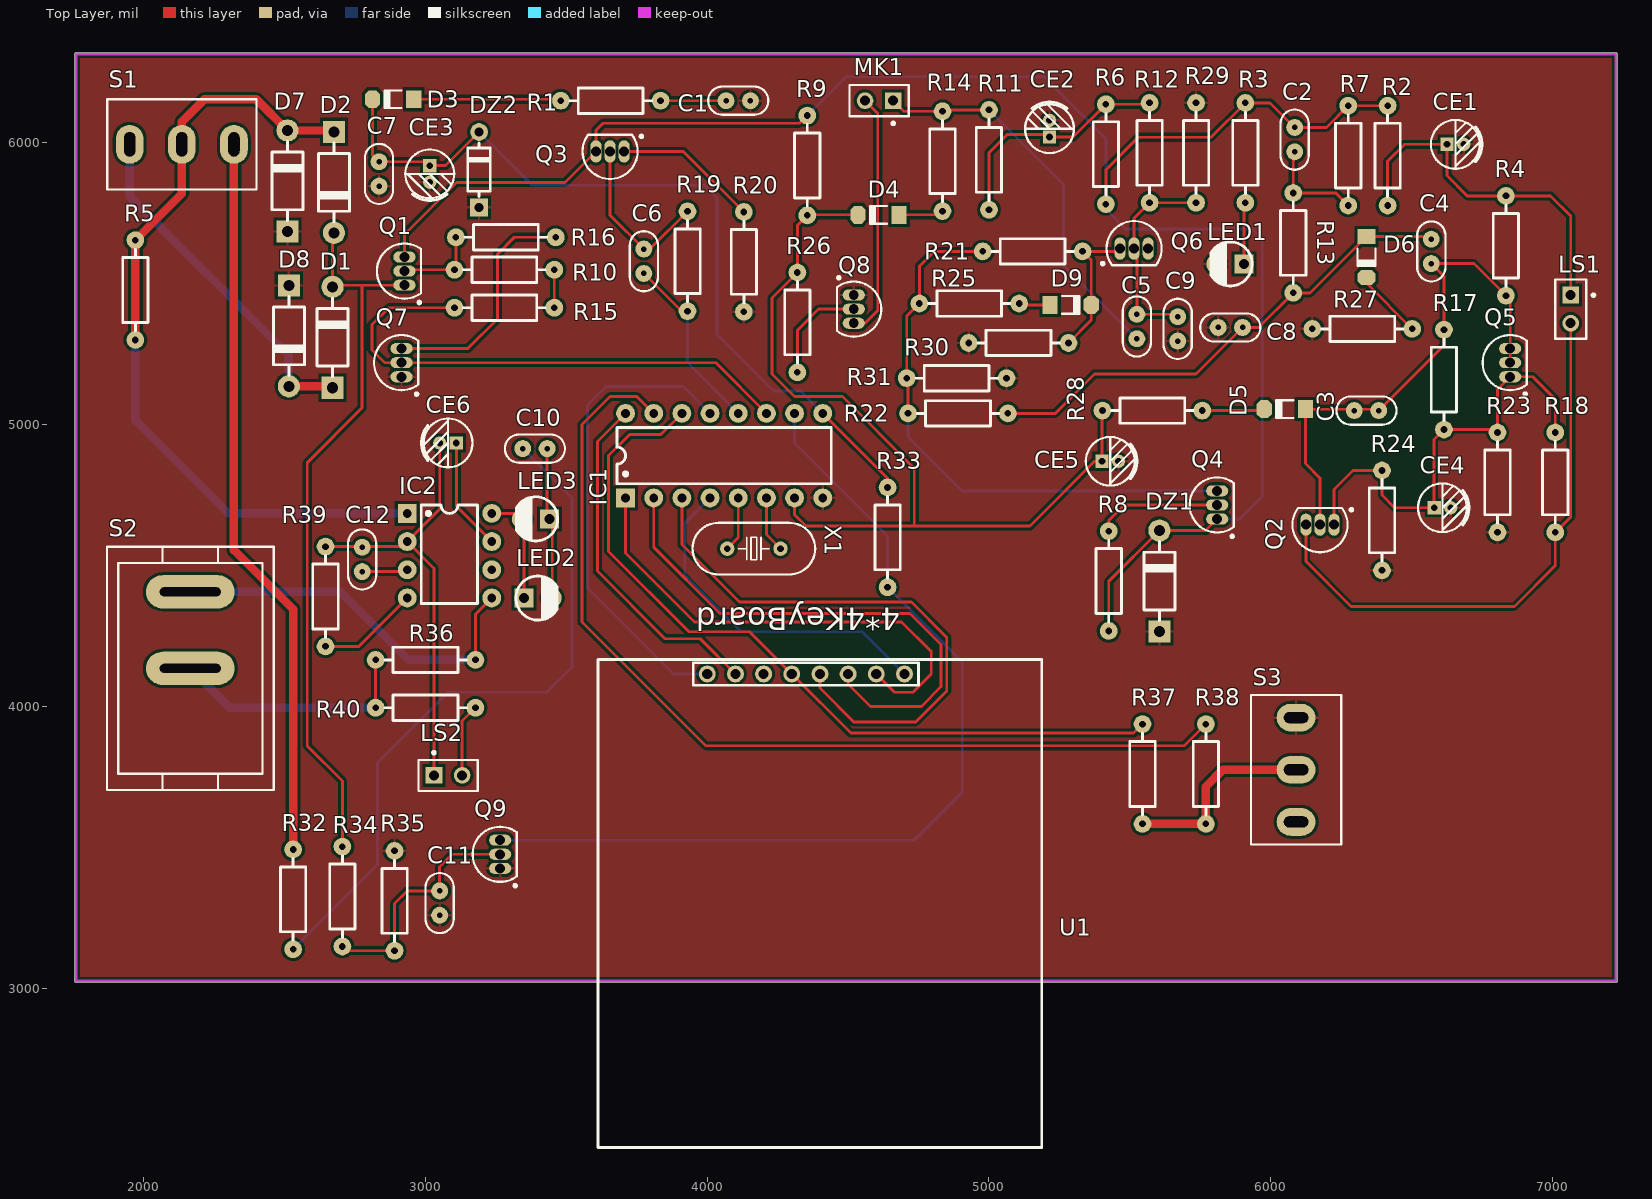
[diagram p0: Top Layer view]
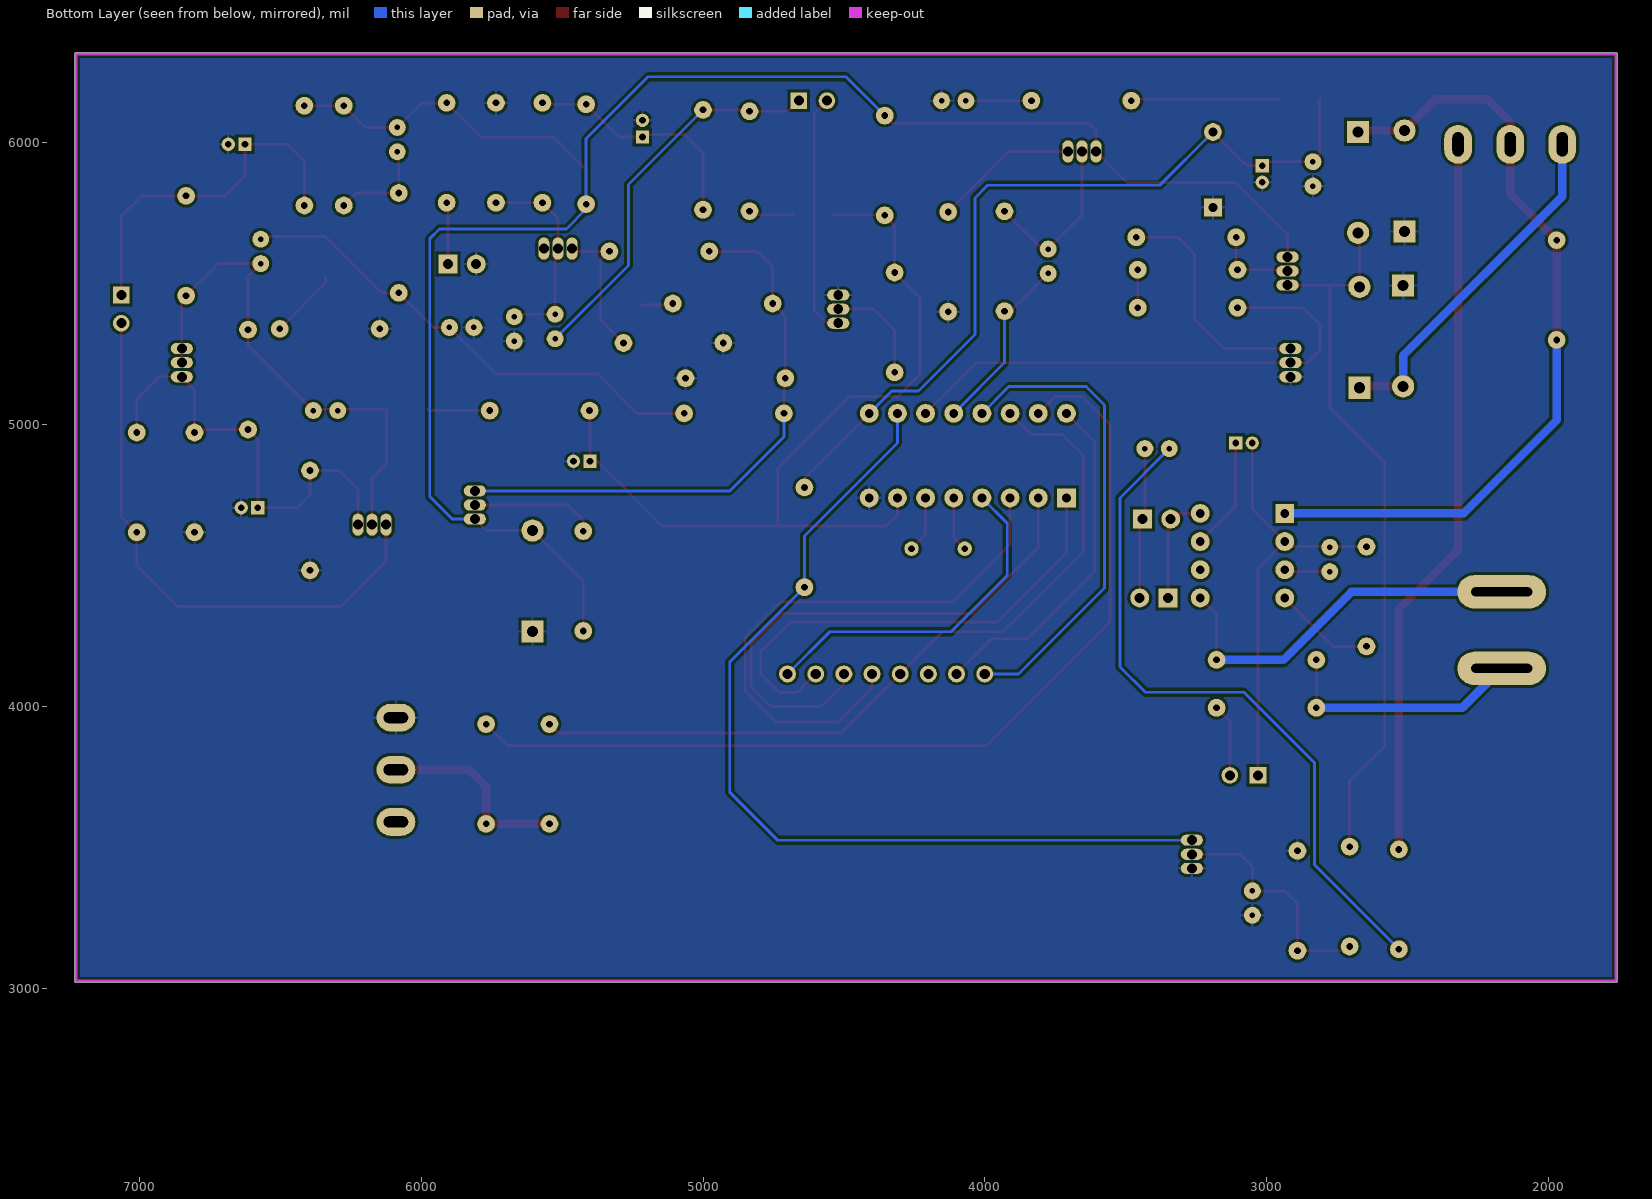
[diagram p1: Bottom Layer view, seen from below]
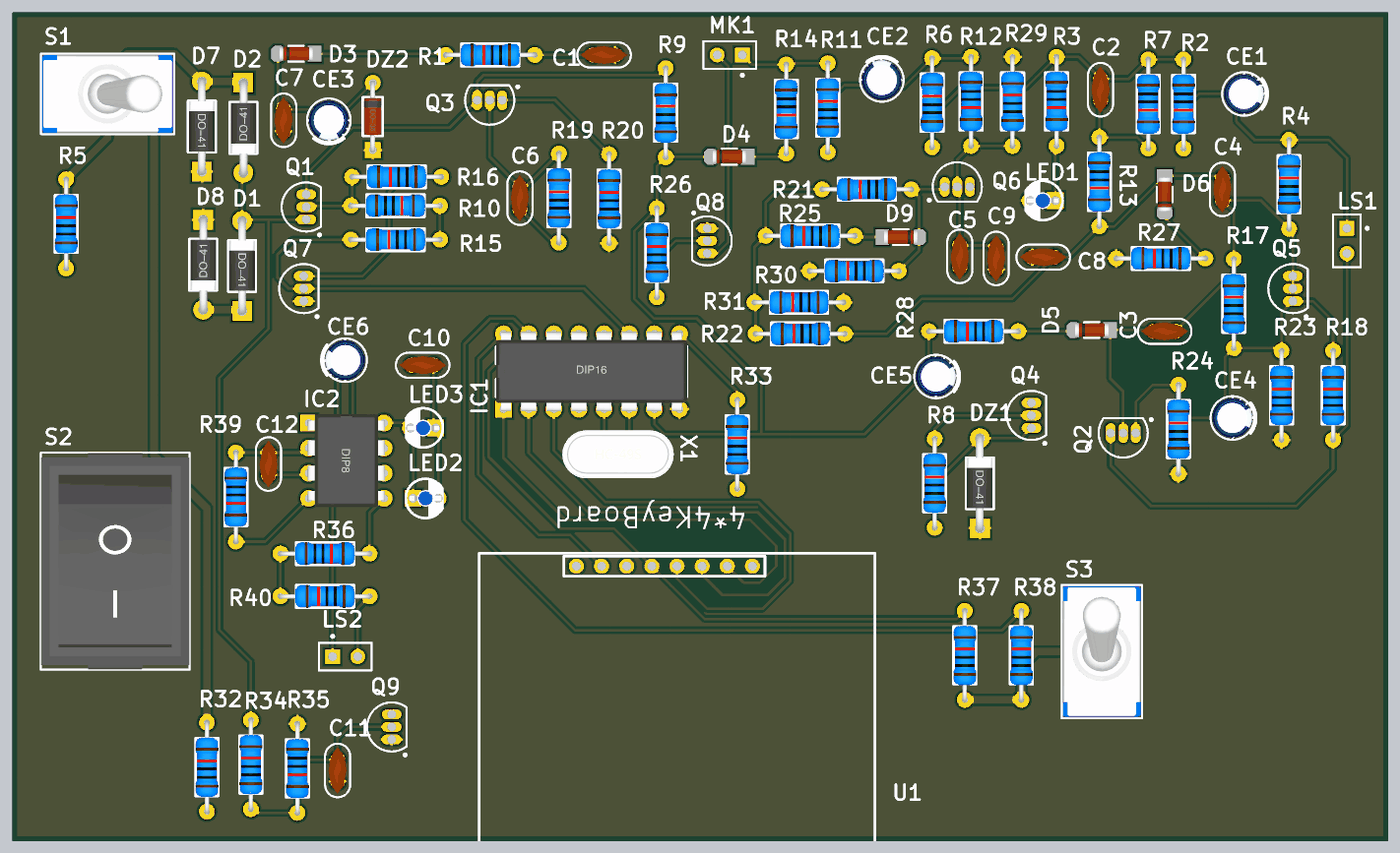
[diagram p2: 3D render of the assembled board from above, using the file's embedded part models]
# Altium PCB MISC82217.PcbDoc
Units mil, origin at the board's own origin, x right, y up, seen from the top; angles counter-clockwise.
Board outline 5475.03 x 3300.03 mil, 2 copper layers (Top Layer, Bottom Layer); 91 components, 60 nets, 219 pads, 0 vias.

## Layer stack, top to bottom (the 12.6 mil dielectric is the usual default, probably not edited)
Top Solder: solder mask 0.4, Solder Resist, Dk 3.5
Top Layer: signal copper 1.4
Dielectric 1: dielectric 12.6, FR-4, Dk 4.8
Bottom Layer: signal copper 1.4
Bottom Solder: solder mask 0.4, Solder Resist, Dk 3.5

## Board outline
1760,3019.99 cw(c1760,3025) 1754.98,3025 1754.98,6315 cw(c1760,6315) 1760,6320.02 7225,6320.02 cw(c7225,6315) 7230.02,6315 7230.02,3025 cw(c7225,3025) 7225,3019.99

## Design rules (kind name [scope] priority, off if disabled: settings)
Clearance [All] p1: gap=10
Height [All] p1: minheight=0 maxheight=99999 prefheight=500
HoleSize [All] p1: absolutevalues=TRUE maxlimit=1000 minlimit=1 maxpercent=80.000 minpercent=20.000
MinimumSolderMaskSliver [All] p1: minsoldermaskwidth=0
PolygonConnect [All] p1: connectstyle=Relief reliefconductorwidth=10 reliefentries=4 polygonreliefangle="90 Angle" airgapwidth=10
RoutingVias [All] p1: holewidth=28 width=50 viastyle="Through Hole" minholewidth=28 minwidth=50 maxholewidth=28 maxwidth=50
SilkToSilkClearance [All] p1: silktosilkclearance=0
SilkToSolderMaskClearance [IsPad] p1: minsilkscreentomaskgap=0 clearancetoexposedcopper=TRUE
SolderMaskExpansion [All] p1: expansion=4
Width [All] p1: maxlimit=30 minlimit=10 preferedwidth=10
25 further rules are at their usual default settings.

## Components (designator, comment, footprint, x,y, rotation, side; value= is the part's Value field where it differs from the comment)
C1 "22NF" "CC 2.2*5" 4110,6150 r180 top
C2 "10NF" "CC 2.2*5" 6085,6011.69 r90 top
C3 "100NF" "CC 2.2*5" 6340,5050 r180 top
C4 "100NF" "CC 2.2*5" 6570,5615 r90 top
C5 "10NF" "CC 2.2*5" 5525,5348.31 r270 top
C6 "22NF" "CC 2.2*5" 3775,5580 r90 top
C7 "100NF" "CC 2.2*5" 2835,5890 r90 top
C8 "22NF" "CC 2.2*5" 5856.69,5345 r0 top
C9 "33NF" "CC 2.2*5" 5670,5340 r90 top
C10 "1UF" "CC 2.2*5" 3388.31,4915 r0 top
C11 "100NF" "CC 2.2*5" 3050,3301.69 r90 top
C12 "100NF" "CC 2.2*5" 2775,4521.69 r270 top
CE1 "100UF" "CAP 1.5*4*8" 6655.47,5995 r0 top
CE2 "4.7UF" "CAP 1.5*4*8" 5215,6050.47 r90 top
CE3 "100UF" "CAP 1.5*4*8" 3015,5890 r270 top
CE4 "47UF" "CAP 1.5*4*8" 6609.53,4705 r0 top
CE5 "4.7UF" "CAP 1.5*4*8" 5430.47,4870 r0 top
CE6 "10uF/16V" "CAP 1.5*4*8" 3080,4935 r180 top
D1 "1N4007" DO-41 2670,5310 r90 top
D2 "1N4007" DO-41 2675,5860 r270 top
D3 "1N4148" "MINI_MELF (LL34)" 2885,6155 r180 top
D4 "1N4148" "MINI_MELF (LL34)" 4608.03,5745 r180 top
D5 "1N4148" "MINI_MELF (LL34)" 6050,5055 r180 top
D6 "1N4148" "MINI_MELF (LL34)" 6340,5595 r270 top
D7 "1N4007" DO-41 2510,5865 r90 top
D8 "1N4007" DO-41 2515,5315 r270 top
D9 "1N4148" "MINI_MELF (LL34)" 5290,5425 r0 top
DZ1 "1N4742" DO-41 5605,4445 r90 top
DZ2 "1N4106" DO-35 3190,5905 r90 top
IC1 "HM91710A" DIP16 4060,4890 r90 top
IC2 "GL6840A" DIP8 3085,4535 r0 top
LED1 "Red" "LED 3MM-B" 5855,5570 r180 top
LED2 "Red" "LED 3MM-B" 3400,4385 r0 top
LED3 "Red" "LED 3MM-B" 3390,4665 r180 top
LS1 "Speaker" PIN2 7065,5460 r270 top
LS2 "Bell" PIN2 3030,3755 r0 top
MK1 "Mic2" PIN2 4660,6150 r180 top
Q1 "A1013" TO-92A 2925,5545 r0 top
Q2 "9014" TO-92A 6175,4645 r90 top
Q3 "5551" TO-92A 3655,5970 r90 top
Q4 "A1013" TO-92A 5810,4715 r0 top
Q5 "9014" TO-92A 6850,5220 r0 top
Q6 "9014" TO-92A 5515,5625 r270 top
Q7 "5551" TO-92A 2915,5220 r0 top
Q8 "5551" TO-92A 4520,5410 r180 top
Q9 "9014" TO-92A 3265,3475 r0 top
R1 "2K2" "RS 1/4W" 3657.17,6150 r180 top
R2 "1K2" "RS 1/4W" 6415,5955 r270 top
R3 "4K7" "RS 1/4W" 5910,5965 r270 top
R4 "10K" "RS 1/4W" 6835,5635 r90 top
R5 "151V" "RS 1/4W" 1970,5477.83 r90 top
R6 "15K" "RS 1/4W" 5415,5960 r90 top
R7 "9K1" "RS 1/4W" 6275,5955 r270 top
R8 "10K" "RS 1/4W" 5425,4445 r90 top
R9 "33K" "RS 1/4W" 4355,5920 r90 top
R10 "100K" "RS 1/4W" 3280,5550 r0 top
R11 "2K" "RS 1/4W" 5000,5940 r90 top
R12 "130K" "RS 1/4W" 5570,5965 r270 top
R13 "5K1" "RS 1/4W" 6080,5645 r270 top
R14 "10K" "RS 1/4W" 4835,5935 r270 top
R15 "200K" "RS 1/4W" 3280,5415 r180 top
R16 "5K1" "RS 1/4W" 3285,5665 r180 top
R17 "20K" "RS 1/4W" 6615,5160 r90 top
R18 "6k2" "RS 1/4W" 7010,4795 r90 top
R19 "5K1" "RS 1/4W" 3930,5580 r90 top
R20 "120" "RS 1/4W" 4130,5577.83 r90 top
R21 "470" "RS 1/4W" 5155,5615 r180 top
R22 "560" "RS 1/4W" 4890,5040 r180 top
R23 "150" "RS 1/4W" 6805,4795 r90 top
R24 "510" "RS 1/4W" 6395,4660 r90 top
R25 "100" "RS 1/4W" 4930,5430 r180 top
R26 "100K" "RS 1/4W" 4320,5362.83 r90 top
R27 "100" "RS 1/4W" 6325,5340 r180 top
R28 "2K" "RS 1/4W" 5580,5050 r180 top
R29 "27K" "RS 1/4W" 5735,5965 r90 top
R30 "75K" "RS 1/4W" 5105,5290 r180 top
R31 "18" "RS 1/4W" 4885,5165 r180 top
R32 "1K5" "RS 1/4W" 2530,3315 r90 top
R33 "470k" "RS 1/4W" 4640,4600 r90 top
R34 "470k" "RS 1/4W" 2705,3325 r90 top
R35 "470k" "RS 1/4W" 2890,3310 r270 top
R36 "7K5" "RS 1/4W" 3000,4165 r0 top
R37 "820K" "RS 1/4W" 5545,3760 r90 top
R38 "820K" "RS 1/4W" 5770,3760 r90 top
R39 "33K" "RS 1/4W" 2645,4390 r270 top
R40 "1K5" "RS 1/4W" 3000,3995 r180 top
S1 "MTS-10x" MTS-10x 2135,5995 r0 top
S2 "KCD1-101" KCD1-101 2165,4135 r90 top
S3 "MTS-10x" MTS-10x 6090,3775 r90 top
U1 "4*4 matrix keypad" "4*4 KEYBOARD" 4400,3389.43 r180 top
X1 "3.58MHZ" "OSC HC-49S" 4165.51,4560 r0 top

## Footprints (in the part's own frame and the unit in brackets; to place one, negate y for a bottom-side part, rotate by r counter-clockwise, add the part's x,y. Pads: shape width x height; smd on the part's side, far side on the other; paste and mask are expansions set on the pad)
"4*4 KEYBOARD" [mil]
  round 60 hole 36 paste+0 mask+2: 1(-300,-725.57) 2(-200,-725.57) 3(-100,-725.57) 4(0,-725.57) 5(100,-725.57) 6(200,-725.57) 7(300,-725.57) 8(400,-725.57)
  silkscreen extent -787,-777 787,956
"CAP 1.5*4*8" [mm] "脚距1.5mm直径4mm高度8mm"
  rect 1.2x1.2 hole 0.6: 1(-0.75,0)
  round 1.2 hole 0.6: 2(0.75,0)
  silkscreen extent -2.2,-2.2 2.41,2.2, body extent -2,-2 2.02,2, height 8.04
"CC 2.2*5" [mil] "脚距2.2mm直径5mm"
  round 60 hole 19.68: 1(-43.31,0) 2(43.31,0)
  silkscreen extent -107,-50 107,50, body extent -94,-36 94,36, height 189
DIP8 [mm]
  rect 1.7x1.7 hole 0.8: 1(-3.81,3.81)
  round 1.7 hole 0.8: 2(-3.81,1.27) 3(-3.81,-1.27) 4(-3.81,-3.81) 5(3.81,-3.81) 6(3.81,-1.27) 7(3.81,1.27) 8(3.81,3.81)
  silkscreen extent -2.54,-4.32 2.54,4.57, body extent -3.94,-4.7 3.91,4.7, height 4.5
DIP16 [mm]
  rect 1.7x1.7 hole 0.8: 1(-3.81,8.89)
  round 1.7 hole 0.8: 2(-3.81,6.35) 3(-3.81,3.81) 4(-3.81,1.27) 5(-3.81,-1.27) 6(-3.81,-3.81) 7(-3.81,-6.35) 8(-3.81,-8.89) 9(3.81,-8.89) 10(3.81,-6.35) 11(3.81,-3.81) 12(3.81,-1.27) 13(3.81,1.27) 14(3.81,3.81) 15(3.81,6.35) 16(3.81,8.89)
  silkscreen extent -2.54,-9.65 2.54,9.65, body extent -4.02,-9.65 4.02,9.65, height 4.45
DO-35 [mm] "1.8*6.8mm(直径，脚距）"
  rect 1.6x1.6 hole 0.8: 1(-3.4,0)
  round 1.6 hole 0.8: 2(3.4,0)
  silkscreen extent -2.41,-1.02 2.41,1.02, body extent -3.65,-0.9 3.65,0.9, height 1.85
DO-41 [mm] "2.6*9.1mm(直径，脚距）"
  rect 2x2 hole 1: 1(-4.55,0)
  round 2 hole 1: 2(4.55,0)
  silkscreen extent -3.56,-1.4 3.56,1.4, body extent -4.92,-1.29 4.98,1.31, height 2.65
KCD1-101 [mm] "船型开关立式"
  oval 3x8 hole 0.8 slot 5.5 at 90 deg: 1(0,0) 2(6.9,0)
  silkscreen extent -10.97,-7.52 10.97,7.52, body extent -10.95,-7.5 10.95,7.5, height 20.3
"LED 3MM-B" [mm] "蓝色3mm直插LED"
  rect 1.7x1.7 hole 0.9: 1(-1.27,0)
  round 1.7 hole 0.9: 2(1.27,0)
  silkscreen extent -2.01,-2 1.72,1.98, body extent -1.95,-1.95 1.64,1.95, height 5.55
"MINI_MELF (LL34)" [mm] "1.5*3.4mm(直径，脚距）"
  rect 1.37x1.62 smd: 1(-1.855,0)
  oct 1.37x1.62 smd: 2(1.855,0)
  silkscreen extent -0.76,-0.8 0.78,0.8, body extent -1.7,-0.75 1.7,0.75, height 1.5
MTS-10x [mm] "MTS10系列3脚扭子开关"
  oval 2.5x3.5 hole 1 slot 2.2 at 90 deg unplated: 1(-4.7,0) 2(0,0) 3(4.7,0)
  silkscreen extent -6.73,-4.06 6.73,4.06, body extent -6.6,-3.95 6.6,3.95, height 30.47
"OSC HC-49S" [mm]
  round 1.3 hole 0.6: 1(-2.4,0) 2(2.4,0)
  silkscreen extent -5.52,-2.32 5.52,2.33, body extent -5.52,-2.32 5.53,2.33, height 4.13
PIN2 [mm] "Photosensitive Diode; 2 Leads"
  rect 1.5x1.5 hole 0.9: 1(0,0)
  round 1.5 hole 0.9: 2(2.54,0)
  silkscreen extent -1.4,-1.4 3.94,2.18
"RS 1/4W" [mm] "直插色环电阻，脚距9mm，直径2.3mm"
  round 1.6 hole 0.6: 1(-4.5,0) 2(4.5,0)
  silkscreen extent -3.68,-1.14 3.68,1.14, body extent -4.72,-1.16 4.73,1.16, height 2.32
TO-92A [mm] "TO, Flat Index; 3 In-Line, Axial Leads; Body Dia. 4.5mm; Leads 0.51 x 0.48 mm (max)"
  oval 2x1 hole 0.9: 1(0,-1.27) 2(0,0) 3(0,1.27)
  silkscreen extent -2.48,-2.95 1.5,2.48, body extent -2.48,-2.5 1.5,2.5, height 6.86

## Part data
C1 C2 C3 C4 C5 C6 C7 C8 C9 C10 C11 C12: library part CC, "Ceramic disc capacitor"
CE1 CE2 CE3 CE4 CE5 CE6: library part CE, "Through-hole electrolytic capacitor"
D1 D2 D7 D8: "Rectifier diode"
D3 D4 D5 D6 D9: "Switching diode"
DZ1: library part 1N4733, "5.1V/1W Zener diode"
DZ2: "12V/0.5W Zener diode"
LED1 LED2 LED3: library part LED-3MM, "Through-hole 3mm LED"
LS1: "Loudspeaker"
LS2: "Electrical Bell"
MK1: "Microphone"
Q1 Q4: library part 2N3906, "PNP General Purpose Amplifier"
Q2 Q3 Q5 Q6 Q7 Q8 Q9: library part 2N3904, "NPN General Purpose Amplifier"
R1 R2 R3 R4 R5 R6 R7 R8 R9 R10 R11 R12 R13 R14 R15 R16 R17 R18 R19 R20 R21 R22 R23 R24 R25 R26 R27 R28 R29 R30 R31 R32 R33 R34 R35 R36 R37 R38 R39 R40: library part R-S, "Color-band resistor"
S1 S3: "MTS10x series 3-pin twist switch"
S2: "1-way SPST boat-type switch"
U1: library part 4*4矩阵键盘
X1: library part XTAL-2P, "2-pin passive crystal"

## Nets (pads, with @x,y where several pads share a name; then routed paths per layer and width w, separated by ;. In a path a pad name is that pad's centre, name@x,y a point inside that pad or via, vN(x,y) a via of type N, cw(c..) or ccw(c..) an arc to the next point about the centre after c; other vN are vias at no path point)
GND: C1.1 C7.1 C8.1 C9.1 C11.1 CE1.2 CE2.2 CE3.2 CE4.2 CE5.2 D7.1 D8.1 DZ1.1 DZ2.1 IC1.8 LED1.2 Q7.1 Q8.1 Q9.1 R20.1 R23.1 R24.1 R27.2 R29.2 R30.2 R31.1 R35.1 S3.3
NetC1_2: C1.2 R1.1 | length 232.4
  Top Layer w10: R1.1 C1.2
NetC2_1: C2.1 R7.2 R13.1 | length 361.7
  Top Layer w10: C2.1 6080,5963.39 R13.1 6230.67,5822.17 R7.2
NetC2_2: C2.2 DZ1.2 Q1.3 Q3.3 Q4.1 R2.1 R3.1 R6.1 R7.1 R8.1 R9.2 | length 6834.9
  Top Layer w10: Q1.3 2925,5675 3110,5860 3495,5860 Q3.3 3605,6045 3630,6070 4327.83,6070 R9.2 ; R6.1 5415,5905 5530,6020 5787.83,6020 R3.1 5997.83,6142.17 C2.2 6197.83,6055 R7.1 R2.1 ; R8.1 5425,4444.13 DZ1.2 5769.13,4624.13 Q4.1
  Bottom Layer w10: R9.2 4492.83,6235 5195,6235 5415,6015 R6.1 5415,5765 5485,5695 5935,5695 5970,5660 5970,4745 5890,4665 Q4.1
NetC3_1: C3.1 C3.2 C4.1 D5.1 Q2.2 Q5.2 Q5.3 R4.1 R17.2 | length 1886.4
  Top Layer w10: Q2.2 6175,4810 6123.03,4861.97 D5.1 6378.31,5055 C3.1 6615,5281.69 R17.2 6615,5526.69 C4.1 6721.14,5571.69 R4.1 6850,5442.83 Q5.3 Q5.2
NetC4_2: C4.2 C8.2 D6.1 R13.2 R22.1 | length 1767
  Top Layer w10: R22.1 5235,5040 5375,5180 5735,5180 C8.2 5957.17,5345 R13.2 6139.8,5467.83 D6.1 6560.28,5668.03 C4.2
NetC5_1: C5.1 C9.2 Q6.2 R12.2 R29.1 | length 739.6
  Top Layer w10: Q6.2 5515,5732.83 R12.2 R29.1 ; Q6.2@5530.31,5630 5525,5624.69 C5.1 5661.69,5391.61 C9.2
NetC5_2: C5.2 MK1.1 R11.2 R14.1 | length 1387.4
  Top Layer w10: MK1.1 4697.83,6112.17 R14.1 4840,6117.17 R11.2
  Bottom Layer w10: R11.2 5265,5852.17 5265,5565 C5.2
NetC6_1: C6.1 IC1.12 R19.1 | length 647.8
  Top Layer w10: C6.1 3908.86,5402.83 R19.1
  Bottom Layer w10: R19.1 3930,5220 IC1.12
NetC6_2: C6.2 Q3.2 R19.2 | length 606.8
  Top Layer w10: Q3.2 3655,5743.31 C6.2 3796.14,5623.31 R19.2
NetC7_2: C7.2 CE3.1 D3.2 DZ2.2 IC1.9 R33.2 | length 2917.3
  Top Layer w10: D3.2 2811.97,5956.34 C7.2 3001.22,5933.31 CE3.1 3070.67,5919.53 DZ2.2 ; IC1.9 4640,4810 R33.2
  Bottom Layer w10: DZ2.2 3378.86,5850 3990,5850 4035,5805 4035,5320 4235,5120 4330,5120 IC1.9
NetC10_1: C10.1 R32.1 | length 2464.7
  Bottom Layer w10: R32.1 2830,3437.83 2830,3800 3080,4050 3430,4050 3520,4140 3520,4740 C10.1
NetC10_2: C10.2 LED2.2 LED3.1 | length 537.6
  Top Layer w10: C10.2 3431.61,4673.39 LED3.1 3450,4655 LED2.2
NetC11_2: C11.2 Q9.2 R34.1 R35.2 | length 855.7
  Top Layer w10: R34.1 2720,3132.83 R35.2 2890,3300 2935,3345 C11.2 3050,3430 3095,3475 Q9.2
NetC12_1: C12.1 CE6.2 IC2.2 LS2.1 R39.1 | length 1564.6
  Top Layer w10: R39.1 2917.17,4567.17 IC2.2 ; LS2.1 3030,4490 IC2.2 ; CE6.2 3050.47,4700.47 IC2.2
NetC12_2: C12.2 IC2.3 | length 162.7
  Top Layer w10: C12.2 2928.39,4478.39 IC2.3
NetCE1_1: CE1.1 LS1.1 R2.2 R4.2 | length 1282.6
  Top Layer w10: R2.2 6415,5935 6475,5995 CE1.1 6625.94,5884.06 6697.83,5812.17 R4.2 6992.83,5812.17 7065,5740 LS1.1
NetCE2_1: CE2.1 R6.2 R11.1 R12.1 | length 853.1
  Top Layer w10: R11.1 5000,5965 5065,6030 5205.94,6030 CE2.1 5298.78,6020.94 R6.2 5565,6137.17 R12.1
NetCE4_1: CE4.1 Q2.1 Q5.1 R17.1 R18.2 R23.2 R24.2 | length 1627.8
  Top Layer w10: Q2.1 6225,4770 6292.17,4837.17 R24.2 6395,4750 6440,4705 CE4.1 6580,4947.83 R17.1 6794.33,4982.83 R23.2 6805,5125 Q5.1 6930,5170 7010,5090 R18.2
NetCE5_1: CE5.1 D4.2 IC1.7 R9.1 R26.2 R28.2 | length 3087.8
  Top Layer w10: IC1.7 4310,4680 4350,4640 4735,4640 ; D4.2 4357.17,5745 R9.1 4320,5707.83 R26.2 4230,5450 4230,5180 4310,5100 4480,5100 4735,4845 4735,4640 ; R28.2 5400.94,5048.11 CE5.1 5375,4870 5145,4640 4735,4640
NetCE6_1: CE6.1 IC2.7 | length 402
  Top Layer w10: CE6.1 3109.53,4710.47 IC2.7
NetD1_1: D1.1 D8.2 S1.1 | length 1250.3
  Top Layer w30: D8.2 2665,5135.87 D1.1
  Bottom Layer w30: S1.1 1949.96,5810.04 2515,5245 D8.2
NetD1_2: D1.2 D2.2 Q1.1 R34.2 | length 2576.6
  Top Layer w10: D2.2 2670,5675.87 D1.2 2675.87,5495 2775,5495 ; R34.2 2705,3735 2580,3860 2580,4865 2775,5060 2775,5495 ; Q1.1 2775,5495
NetD2_1: D2.1 D7.2 IC2.1 R5.1 R5.2 S1.2 | length 2851.2
  Top Layer w30: R5.1 R5.2 2135,5820 S1.2 2135,6075 2215,6155 2399.13,6155 D7.2 2670,6044.13 D2.1
  Bottom Layer w30: R5.1 1970,5015 2300,4685 IC2.1
NetD3_1: D3.1 R1.2 | length 524
  Top Layer w10: D3.1 3475,6155 R1.2
NetD4_1: D4.1 R14.2 | length 159.3
  Top Layer w10: D4.1 4822.17,5745 R14.2
NetD5_2: D5.2 R28.1 | length 221.9
  Top Layer w10: R28.1 5971.97,5050 D5.2
NetD6_2: D6.2 R27.1 | length 249.1
  Top Layer w10: D6.2 6340,5502.17 R27.1
NetD9_1: D9.1 R25.1 | length 111.9
  Top Layer w10: R25.1 5112.17,5425 D9.1
NetD9_2: D9.2 Q6.1 R21.1 R30.1 | length 508.3
  Top Layer w10: R30.1 5363.03,5370.87 D9.2 5363.03,5584.13 R21.1 5455,5615 Q6.1
NetIC1_1: IC1.1 U1.2 | length 1753.8
  Top Layer w10: IC1.1 3710,4545 3955,4300 4690,4300 4795,4195 4795,4115 4730,4050 4665,4050 U1.2
NetIC1_2: IC1.2 U1.3 | length 1915
  Top Layer w10: IC1.2 3810,4565 4045,4330 4720,4330 4830,4220 4830,4070 4760,4000 4580,4000 4500,4080 U1.3
NetIC1_3: IC1.3 U1.4 | length 2027
  Top Layer w10: IC1.3 3910,4575 4115,4370 4725,4370 4850,4245 4850,4055 4740,3945 4520,3945 4400,4065 U1.4
NetIC1_4: IC1.4 U1.1 | length 1237.3
  Bottom Layer w10: IC1.4 3920,4650 3920,4465 4120,4265 4550,4265 U1.1
NetIC1_5: IC1.5 X1.1 | length 196.1
  Top Layer w10: X1.1 4110,4598.98 IC1.5
NetIC1_6: IC1.6 X1.2 | length 200.7
  Top Layer w10: IC1.6 4210,4610 X1.2
NetIC1_10: IC1.10 Q9.3 R33.1 | length 3301.9
  Bottom Layer w10: Q9.3 4735,3525 4905,3695 4905,4157.83 R33.1 4640,4605 4310,4935 IC1.10
NetIC1_11: IC1.11 Q7.2 R15.2 | length 1900.9
  Top Layer w10: R15.2 2870,5415 2810,5355 2810,5265 2855,5220 Q7.2 4030,5220 IC1.11
NetIC1_13: IC1.13 U1.8 | length 1702.6
  Bottom Layer w10: U1.8 3880,4115 3575,4420 3575,5070 3640,5135 3915,5135 IC1.13
NetIC1_14: IC1.14 R37.2 U1.5 | length 2837.6
  Top Layer w10: IC1.14 3835,4965 3725,4965 3650,4890 3650,4550 3935,4265 4150,4265 U1.5 4510,3905 5512.83,3905 R37.2
NetIC1_15: IC1.15 R38.2 | length 3450.5
  Top Layer w10: IC1.15 3750,5100 3655,5100 3555,5000 3555,4300 3995,3860 5692.83,3860 R38.2
NetIC1_16: IC1.16 U1.7 | length 1242.6
  Top Layer w10: IC1.16 3610,4940 3610,4480 3850,4240 3975,4240 U1.7
NetIC2_4: IC2.4 R39.2 | length 361.3
  Top Layer w10: R39.2 2762.83,4212.83 IC2.4
NetIC2_5: IC2.5 R36.2 S2.2 | length 1356.2
  Top Layer w10: R36.2 3177.17,4327.17 IC2.5
  Bottom Layer w30: S2.2 2698.35,4406.65 2940,4165 R36.2
NetIC2_8: IC2.8 LED2.1 LED3.2 | length 397.4
  Top Layer w10: IC2.8 3320,4685 LED3.2 3350,4655 LED2.1
NetLED1_1: LED1.1 R3.2 | length 219.9
  Top Layer w10: LED1.1 5905,5782.83 R3.2
NetLS1_2: LS1.2 Q2.3 R18.1 | length 2024.1
  Top Layer w10: Q2.3 6125,4515 6285,4355 6865,4355 7010,4500 R18.1 7065,4672.83 LS1.2
NetLS2_2: LS2.2 R40.1 | length 259.5
  Top Layer w10: LS2.2 3130,3947.83 R40.1
NetMK1_2: MK1.2 Q8.3 | length 867.3
  Top Layer w10: Q8.3 4560,5360 4605,5405 4605,6105 MK1.2
NetQ1_2: Q1.2 R10.1 R16.2 | length 297
  Top Layer w10: Q1.2 2930,5550 R10.1 3107.83,5555 R16.2
NetQ3_1: Q3.1 R20.2 | length 514.1
  Top Layer w10: Q3.1 3915,5970 R20.2
NetQ4_2: Q4.2 R8.2 | length 445.6
  Top Layer w10: R8.2 5425,4660 5480,4715 Q4.2
NetQ4_3: Q4.3 R21.2 R22.2 R25.2 R31.2 | length 2049.4
  Top Layer w10: R22.2 4712.83,5160 R31.2 4707.83,5385 R25.2 4752.83,5562.17 4805.67,5615 R21.2
  Bottom Layer w10: R22.2 4712.83,4957.17 4905,4765 Q4.3
NetQ7_3: Q7.3 R16.1 | length 845.5
  Top Layer w10: Q7.3 3150,5270 3255,5375 3255,5605 3315,5665 R16.1
NetQ8_2: Q8.2 R26.1 | length 380.4
  Top Layer w10: R26.1 4320,5335 4395,5410 Q8.2
NetR10_2: R10.2 R15.1 | length 135
  Top Layer w10: R15.1 R10.2
NetR32_2: R32.2 S1.3 | length 2589.8
  Top Layer w30: S1.3 2320.04,4554.96 2530,4345 R32.2
NetR36_1: R36.1 R40.2 S2.1 | length 885.8
  Top Layer w10: R40.2 R36.1
  Bottom Layer w30: S2.1 2305,3995 R40.2
NetR37_1: R37.1 R38.1 S3.2 | length 702
  Top Layer w30: R37.1 R38.1 5770,3715 5830,3775 S3.2
VCC: S3.1
pads on no net: IC2.6 Q6.3 U1.6

## Polygon pours and split planes (outlines as drawn)
GND on Top Layer "D" (solid, remove dead copper, pour order 6): 1465,6480 7400,6480 7420,6500 7420,2785 1490,2785 1450,2745
GND on Bottom Layer "D" (solid, remove dead copper, pour order 8): 1215,6525 1270,6470 7700,6470 7700,2850 7500,2650 7440,2590 1005,2590

## Keep-outs
Keep-Out Layer:
  lines w10: 7225,3270 7225,6315 1760,6315 1760,3025 7225,3025 7225,3280